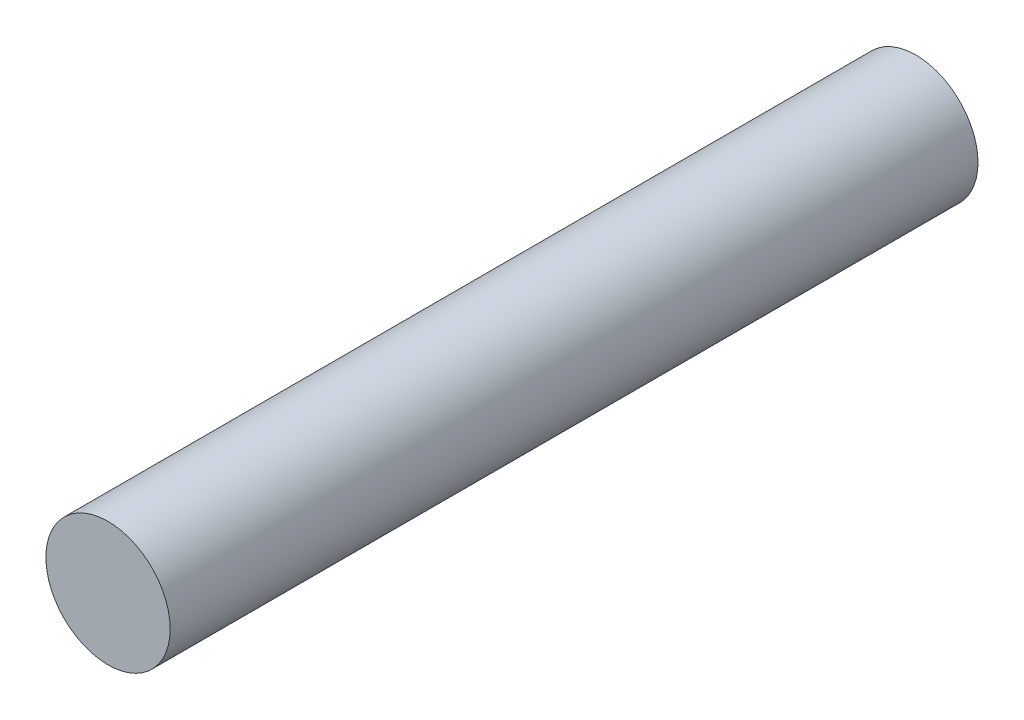
SolidWorks part; units mm, degrees
ref_plane "前视基准面" through (0, 0, 0) normal (0, 0, 1) x (1, 0, 0)
ref_plane "上视基准面" through (0, 0, 0) normal (0, 1, 0) x (1, 0, 0)
ref_plane "右视基准面" through (0, 0, 0) normal (1, 0, 0) x (0, 0, -1)
sketch "草图1" plane through (0, 0, 0) normal (0, 0, 1) x (1, 0, 0)
  circle A0 centre (0, 0) radius 10
  dimension "D1" = 20
extrude "凸台-拉伸1" add sketch "草图1" along normal blind 130
